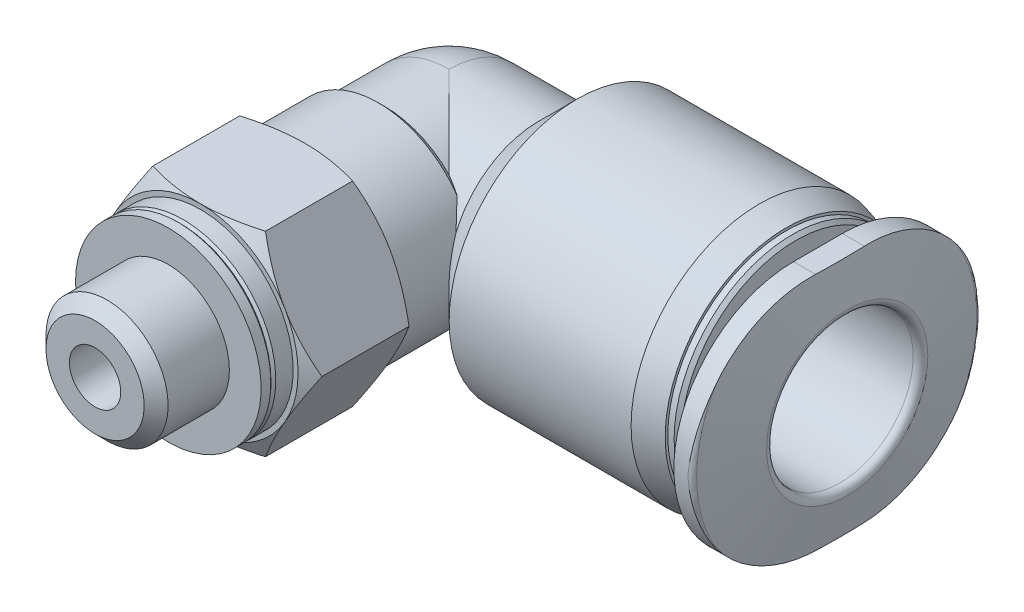
from build123d import *

# Parameters (mm, degrees)
CUT_EXTRUDE1_DEPTH = 1.2
SKETCH6_W          = 14.5
SKETCH6_H          = 1.05
SKETCH7_W          = 16
SKETCH7_H          = 16
CUT_EXTRUDE2_DEPTH = 5.666666667


with BuildPart() as part:
    # Sketch1 → Revolve1 (revolve)
    with BuildSketch(Plane.XY, mode=Mode.PRIVATE) as revolve1_sk:
        with BuildLine():
            Line((0, 3.675), (3.675, 3.675))
            Line((3.675, 3.675), (5.25, 5.25))
            Line((5.25, 5.25), (12.7, 5.25))
            Line((12.7, 5.25), (13.8, 4.955255888))
            Line((13.8, 4.955255888), (13.8, 4.848076211))
            Line((13.8, 4.848076211), (14.058578644, 4.848076211))
            Line((14.058578644, 4.848076211), (14.2, 4.706654855))
            Line((14.2, 4.706654855), (14.2, 3.5))
            Line((14.2, 3.5), (14.73, 3.5))
            ThreePointArc((14.73, 3.5), (14.991629509, 3.608370491), (15.1, 3.87))
            Line((15.1, 3.87), (15.1, 5.9))
            Line((15.1, 5.9), (15.673729924, 5.9))
            ThreePointArc((15.673729924, 5.9), (15.802287446, 5.853208889), (15.870691475, 5.734729636))
            Line((15.870691475, 5.734729636), (16.3, 3.3))
            Line((16.3, 3.3), (16.3, 0))
            Line((16.3, 0), (-3.675, 0))
            ThreePointArc((-3.675, 0), (-2.598617421, 2.598617421), (0, 3.675))
        make_face()
    revolve(revolve1_sk.sketch.rotate(Axis((16.3, 0, 0), (-1, 0, 0)), 90), axis=Axis((16.3, 0, 0), (-1, 0, 0)))

    # Sketch2 → Revolve2 (revolve)
    with BuildSketch(Plane(origin=(0, 0, 0), x_dir=(0, 0, -1), z_dir=(1, 0, 0)), mode=Mode.PRIVATE) as revolve2_sk:
        Polygon((-11.5, 0), (-11.5, 3.8), (-11.1, 3.8), (-11, 3.7), (-10.9, 3.8), (-10.1875, 3.8), (-10.1875, 4), (-9.817995828, 4.64), (-6.275754172, 4.64), (-5.90625, 4), (-5.90625, 3.9375), (-2.9, 3.9375), (-2.6375, 3.675), (0, 3.675), (0, 0), align=None)
    revolve(revolve2_sk.sketch.rotate(Axis((0, 0, 0), (0, 0, 1)), 90), axis=Axis((0, 0, 0), (0, 0, 1)))

    # Sketch3 → Revolve3 (revolve)
    with BuildSketch(Plane(origin=(0, 0, 0), x_dir=(0, 0, -1), z_dir=(1, 0, 0)), mode=Mode.PRIVATE) as revolve3_sk:
        Polygon((-14.5, 0), (-14.5, 2.0095), (-14.0095, 2.5), (-11.5, 2.5), (-11.5, 0), align=None)
    revolve(revolve3_sk.sketch.rotate(Axis((0, 0, 11.5), (0, 0, 1)), 90), axis=Axis((0, 0, 11.5), (0, 0, 1)))

    # Sketch4 → Cut-Extrude1 (cut)
    with BuildSketch(Plane(origin=(16.3, 0, 0), x_dir=(0, 0, -1), z_dir=(1, 0, 0))):
        Polygon((-7.08, 4.087639906), (-7.08, -4.087639906), (0, -8.175279812), (7.08, -4.087639906), (7.08, 4.087639906), (0, 8.175279812), align=None)
        with BuildLine():
            Line((-1, -4.9), (1, -4.9))
            ThreePointArc((1, -4.9), (5.9, 0), (1, 4.9))
            Line((1, 4.9), (-1, 4.9))
            ThreePointArc((-1, 4.9), (-5.9, 0), (-1, -4.9))
        make_face(mode=Mode.SUBTRACT)
    extrude(amount=-CUT_EXTRUDE1_DEPTH, mode=Mode.SUBTRACT)

    # Sketch6 → Cut-Revolve1 (revolve, cut)
    with BuildSketch(Plane(origin=(0, 0, 0), x_dir=(0, 0, -1), z_dir=(1, 0, 0)), mode=Mode.PRIVATE) as cut_revolve1_sk:
        with Locations((-7.25, 0.525)):
            Rectangle(SKETCH6_W, SKETCH6_H)
    revolve(cut_revolve1_sk.sketch.rotate(Axis((0, 0, 0), (0, 0, 1)), 90), axis=Axis((0, 0, 0), (0, 0, 1)), mode=Mode.SUBTRACT)

    # Sketch5 → Cut-Revolve2 (revolve, cut)
    with BuildSketch(Plane(origin=(0, 0, 0), x_dir=(1, 0, 0), z_dir=(0, 1, 0))):
        with BuildLine():
            Line((0, 1.05), (4.4, 1.05))
            Line((4.4, 1.05), (4.4, 3))
            Line((4.4, 3), (16, 3))
            ThreePointArc((16, 3), (16.212132034, 3.087867966), (16.3, 3.3))
            Line((16.3, 3.3), (16.3, 0))
            Line((16.3, 0), (-1.05, 0))
            ThreePointArc((-1.05, 0), (-0.74246212, 0.74246212), (0, 1.05))
        make_face()
    revolve(axis=Axis((16.3, 0, 0), (-1, 0, 0)), mode=Mode.SUBTRACT)

    # Sketch7 → Cut-Extrude2 (cut)
    with BuildSketch(Plane.XY.offset(11.5)):
        Rectangle(SKETCH7_W, SKETCH7_H)
        Polygon((-4.618802154, 0), (-2.309401077, -4), (2.309401077, -4), (4.618802154, 0), (2.309401077, 4), (-2.309401077, 4), align=None, mode=Mode.SUBTRACT)
    extrude(amount=-CUT_EXTRUDE2_DEPTH, mode=Mode.SUBTRACT)


solid = part.part
